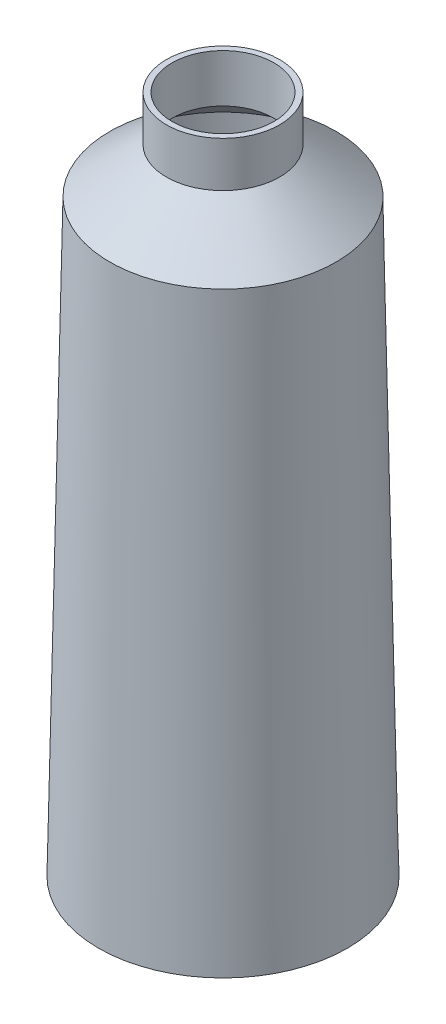
SolidWorks part; units mm, degrees
ref_plane "Front Plane" through (0, 0, 0) normal (0, 0, 1) x (1, 0, 0)
ref_plane "Top Plane" through (0, 0, 0) normal (0, 1, 0) x (1, 0, 0)
ref_plane "Right Plane" through (0, 0, 0) normal (1, 0, 0) x (0, 0, -1)
sketch "Sketch1" plane through (0, 0, 0) normal (0, 0, 1) x (1, 0, 0)
  line L0 (0, 0) -> (0, 300)
  line L1 (0, 300) -> (25, 300)
  line L2 (25, 300) -> (25, 280)
  line L3 (25, 280) -> (50, 260)
  line L4 (50, 260) -> (55, 0)
  line L5 (55, 0) -> (0, 0)
  dimension "D1" = 55
  dimension "D2" = 300
  dimension "D3" = 20
  dimension "D4" = 25
  dimension "D5" = 40
  dimension "D6" = 25
revolve "Revolve1" add sketch "Sketch1" angle 360 about L0
shell "Shell1" thickness 2.5
